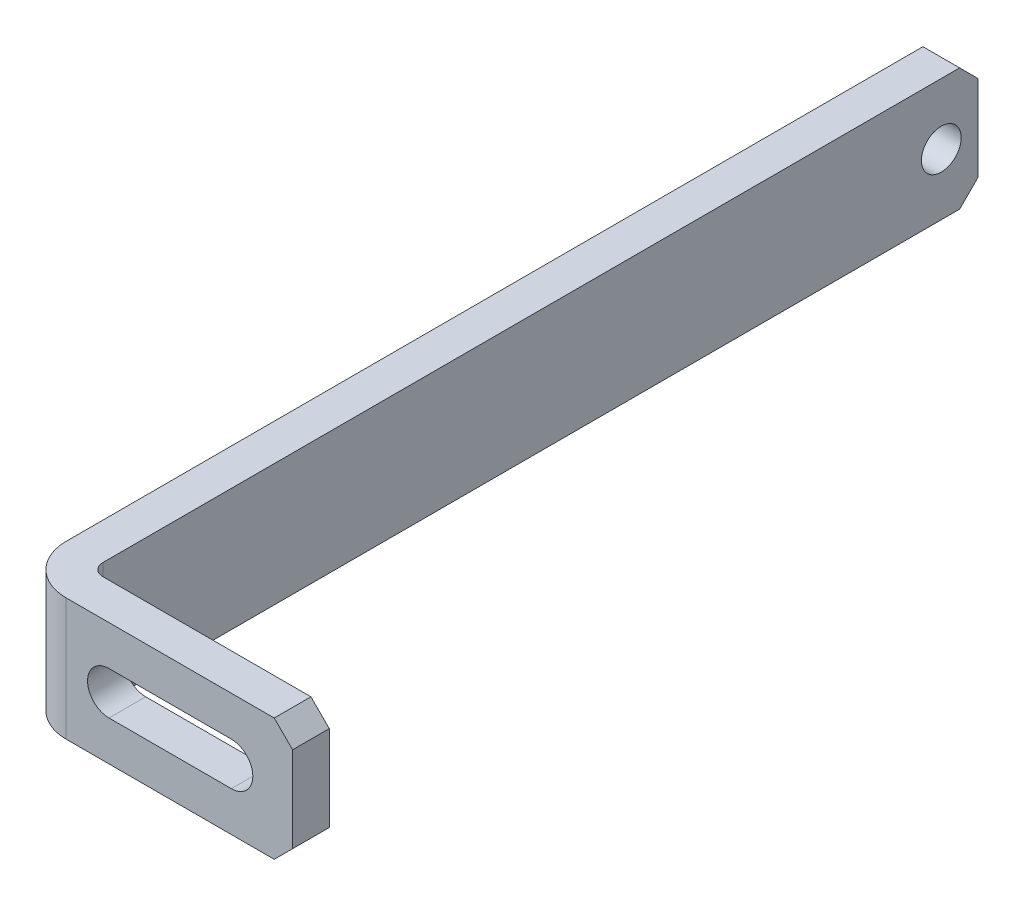
SolidWorks part; units mm, degrees
ref_plane "Front Plane" through (0, 0, 0) normal (0, 0, 1) x (1, 0, 0)
ref_plane "Top Plane" through (0, 0, 0) normal (0, 1, 0) x (1, 0, 0)
ref_plane "Right Plane" through (0, 0, 0) normal (1, 0, 0) x (0, 0, -1)
sketch "Sketch1" plane through (0, 0, 0) normal (0, 1, 0) x (1, 0, 0)
  line L1 (22.5, -75.5) -> (-22.5, -75.5)
  line L2 (22.5, -75.5) -> (22.5, 75.5)
  line L3 (22.5, 75.5) -> (-22.5, 75.5)
  line L4 (-22.5, -75.5) -> (-22.5, 75.5)
  line L5 (22.5, -75.5) -> (-22.5, 75.5) construction
  line L6 (22.5, 75.5) -> (-22.5, -75.5) construction
  point P0 (0, 0)
  dimension "D1" = 151
  dimension "D2" = 45
extrude "Boss-Extrude1" add sketch "Sketch1" along normal blind 20
sketch "Sketch2" plane through (0, 20, 0) normal (0, 1, 0) x (1, 0, 0)
  line L0 (-22.5, 75.5) -> (-22.5, -75.5) construction
  line L1 (22.5, 75.5) -> (-16.5, 75.5)
  line L2 (22.5, 75.5) -> (22.5, -69.5)
  line L3 (22.5, -69.5) -> (-16.5, -69.5)
  line L4 (-16.5, 75.5) -> (-16.5, -69.5)
  line L5 (-22.5, -75.5) -> (22.5, -75.5) construction
  dimension "D1" = 6
  dimension "D2" = 6
extrude "Cut-Extrude1" cut sketch "Sketch2" against normal through all
sketch "Sketch3" plane through (-16.5, 0, 0) normal (1, 0, 0) x (0, 0, -1)
  line L0 (75.5, 0) -> (75.5, 20) construction
  line L1 (75.5, 20) -> (-69.5, 20) construction
  circle A0 centre (69.5, 10) radius 3.25
  dimension "D3" = 6.5
  dimension "D1" = 6
  dimension "D2" = 10
extrude "Cut-Extrude2" cut sketch "Sketch3" against normal through all
sketch "Sketch4" plane through (0, 0, 69.5) normal (0, 0, -1) x (-1, 0, 0)
  line L0 (-12.5, 10) -> (7.5, 10) construction
  line L1 (-12.5, 13.5) -> (7.5, 13.5)
  line L2 (-12.5, 6.5) -> (7.5, 6.5)
  line L3 (16.5, 0) -> (-22.5, 0) construction
  line L4 (-22.5, 0) -> (-22.5, 20) construction
  arc A0 (-12.5, 13.5) -> (-12.5, 6.5) centre (-12.5, 10) ccw
  arc A1 (7.5, 6.5) -> (7.5, 13.5) centre (7.5, 10) ccw
  point P2 (-2.5, 10)
  dimension "D1" = 7
  dimension "D2" = 10
  dimension "D3" = 20
  dimension "D4" = 10
extrude "Cut-Extrude3" cut sketch "Sketch4" against normal through all
chamfer "Chamfer1" distance 3 angle 45 4 edges at (22.5, 0, 72.5) (22.5, 20, 72.5) (-19.5, 0, -75.5) (-19.5, 20, -75.5)
fillet "Fillet1" radius 2 1 edges at (-16.5, 10, 69.5)
fillet "Fillet2" radius 8 1 edges at (-22.5, 10, 75.5)
